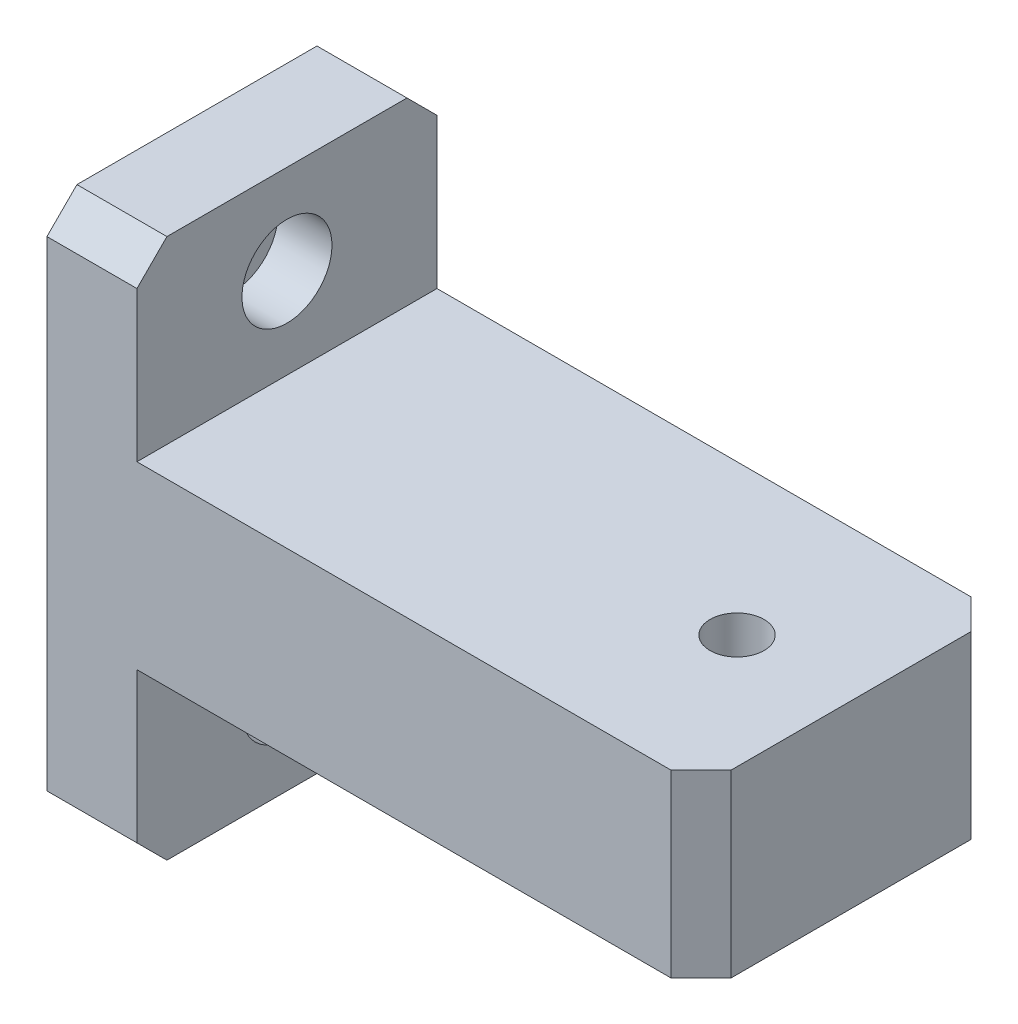
from build123d import *

# Parameters (mm, degrees)
SKETCH_1_W                = 100
SKETCH_1_H                = 30
EXTRUDE_1_DEPTH           = 14
SKETCH_2_W                = 50
SKETCH_2_H                = 30
EXTRUDE_2_DEPTH           = 95
SKETCH_3_R                = 12.5
CUT_EXTRUDE_1_DEPTH       = 5
HOLE_WIZARD_9_0_9_1_D     = 9
HOLE_WIZARD_9_0_9_2_D     = 9
SKETCH_8_OUTSIDE_W        = 132.186
SKETCH_8_OUTSIDE_H        = 62.186
SKETCH_8_OUTSIDE_W_2      = 50
SKETCH_8_OUTSIDE_H_2      = 30
CUT_EXTRUDE_2_DEPTH       = 121.855285362
SKETCH_9_W                = 15
SKETCH_9_H                = 50
EXTRUDE_3_DEPTH           = 30
SKETCH_10_W               = 15
SKETCH_10_H               = 50
EXTRUDE_4_DEPTH           = 30
HOLE_WIZARD_1_D           = 9
HOLE_WIZARD_1_CBORE_D     = 15
HOLE_WIZARD_1_CBORE_DEPTH = 9
CHAMFER_1_SIZE            = 5


with BuildPart() as part:
    # 草图1 → 凸台-拉伸1 (new body)
    with BuildSketch(Plane(origin=(0, 0, 0), x_dir=(0, 0, -1), z_dir=(1, 0, 0))):
        Rectangle(SKETCH_1_W, SKETCH_1_H)
    extrude(amount=EXTRUDE_1_DEPTH)

    # 草图2 → 凸台-拉伸2 (add)
    with BuildSketch(Plane(origin=(14, 0, 0), x_dir=(0, 0, -1), z_dir=(1, 0, 0))):
        Rectangle(SKETCH_2_W, SKETCH_2_H)
    extrude(amount=EXTRUDE_2_DEPTH)

    # 草图3 → 切除-拉伸1 (cut)
    with BuildSketch(Plane.XZ.offset(15)):
        with Locations(Location((90, 0, 0), (0, 0, 270))):
            Circle(SKETCH_3_R)
    extrude(amount=-CUT_EXTRUDE_1_DEPTH, mode=Mode.SUBTRACT)

    # Ø9.0 (9) 直径孔1 (through all)
    with Locations(Plane(origin=(0, -15, 0), x_dir=(-1, 0, 0), z_dir=(0, -1, 0))):
        with Locations((-90, 0)):
            Hole(HOLE_WIZARD_9_0_9_1_D / 2)

    # Ø9.0 (9) 直径孔2 (through all)
    with Locations(Plane(origin=(14, 0, 0), x_dir=(0, 0, -1), z_dir=(1, 0, 0))):
        with Locations((-40, 0), (40, 0)):
            Hole(HOLE_WIZARD_9_0_9_2_D / 2)

    # 草图8 outside → 切除-拉伸2 (cut, through all)
    with BuildSketch(Plane(origin=(109, 0, 0), x_dir=(0, 0, -1), z_dir=(1, 0, 0))):
        Rectangle(SKETCH_8_OUTSIDE_W, SKETCH_8_OUTSIDE_H)
        Rectangle(SKETCH_8_OUTSIDE_W_2, SKETCH_8_OUTSIDE_H_2, mode=Mode.SUBTRACT)
    extrude(amount=-CUT_EXTRUDE_2_DEPTH, mode=Mode.SUBTRACT)

    # 草图9 → 凸台-拉伸3 (add)
    with BuildSketch(Plane.XZ.offset(15)):
        with Locations((7.5, 0)):
            Rectangle(SKETCH_9_W, SKETCH_9_H)
    extrude(amount=EXTRUDE_3_DEPTH)

    # 草图10 → 凸台-拉伸4 (add)
    with BuildSketch(Plane(origin=(0, 15, 0), x_dir=(1, 0, 0), z_dir=(0, 1, 0))):
        with Locations((7.5, 0)):
            Rectangle(SKETCH_10_W, SKETCH_10_H)
    extrude(amount=EXTRUDE_4_DEPTH)

    # 打孔尺寸(%根据)内六角圆柱头螺钉的类型1 (through all)
    with Locations(Plane(origin=(15, 0, 0), x_dir=(0, 0, -1), z_dir=(1, 0, 0))):
        with Locations((0, 30), (0, -30)):
            CounterBoreHole(HOLE_WIZARD_1_D / 2, HOLE_WIZARD_1_CBORE_D / 2, HOLE_WIZARD_1_CBORE_DEPTH)

    # 倒角1
    chamfer_1_edges = [part.edges().sort_by_distance(p)[0] for p in [
        (109, 0, -25),
        (109, 0, 25),
        (7.5, -45, -25),
        (7.5, -45, 25),
        (7.5, 45, 25),
        (7.5, 45, -25),
    ]]
    chamfer(chamfer_1_edges, length=CHAMFER_1_SIZE)


solid = part.part
